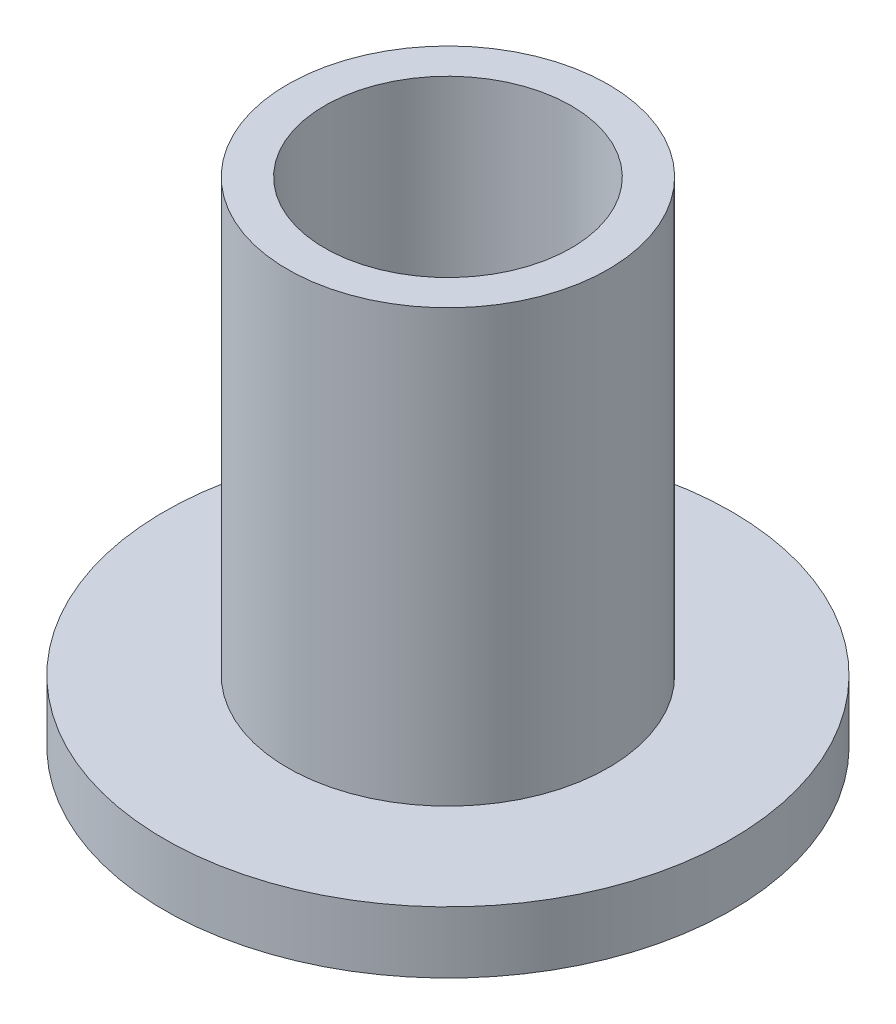
from build123d import *


with BuildPart() as part:
    # 草图1 → 旋转1 (revolve)
    with BuildSketch(Plane.XY, mode=Mode.PRIVATE) as revolve_1_sk:
        Polygon((-10, 0), (-23, 0), (-23, 5), (-13, 5), (-13, 40), (-10, 40), align=None)
    revolve(revolve_1_sk.sketch.rotate(Axis((0, 0, 0), (0, 1, 0)), 270), axis=Axis((0, 0, 0), (0, 1, 0)))


solid = part.part
